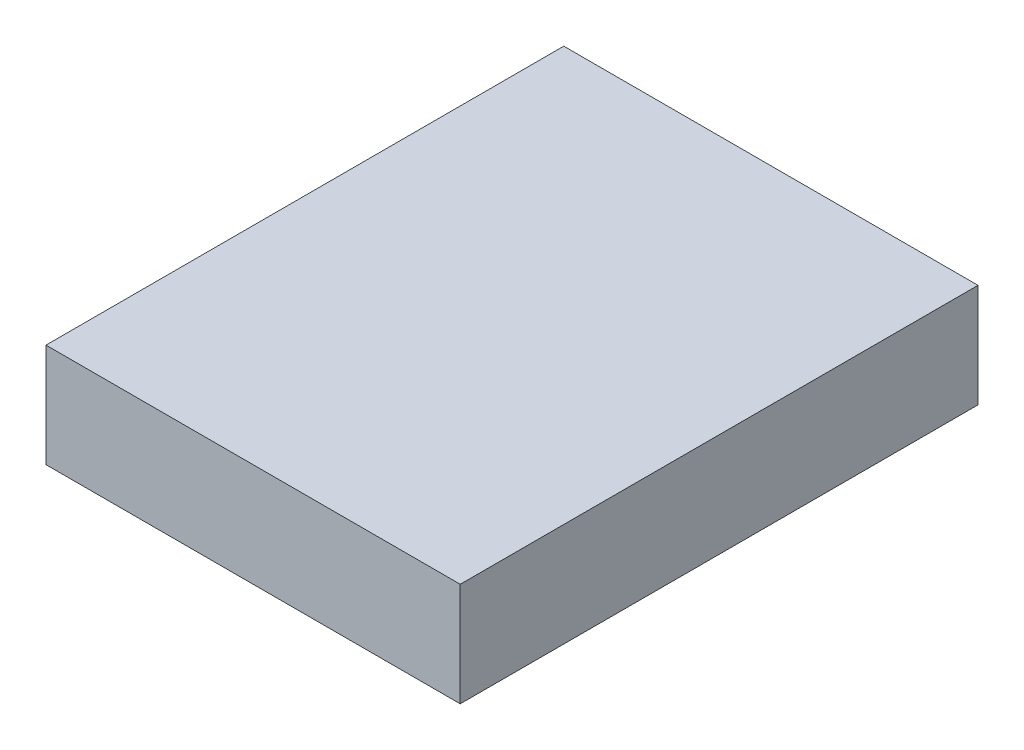
SolidWorks part; units mm, degrees
material "普通碳钢"
ref_plane "Front Plane" through (0, 0, 0) normal (0, 0, 1) x (1, 0, 0)
ref_plane "Top Plane" through (0, 0, 0) normal (0, 1, 0) x (1, 0, 0)
ref_plane "Right Plane" through (0, 0, 0) normal (1, 0, 0) x (0, 0, -1)
sketch "Sketch1" plane through (0, 0, 0) normal (0, 1, 0) x (1, 0, 0)
  line L0 (24, -30) -> (24, 30)
  line L1 (24, 30) -> (-24, 30)
  line L2 (-24, 30) -> (-24, -30)
  line L3 (-24, -30) -> (24, -30)
  point P3 (0, 30)
  point P5 (-24, 0)
  dimension "D1" = 60
  dimension "D2" = 48
extrude "Extrude1" add sketch "Sketch1" along normal mid plane 12
